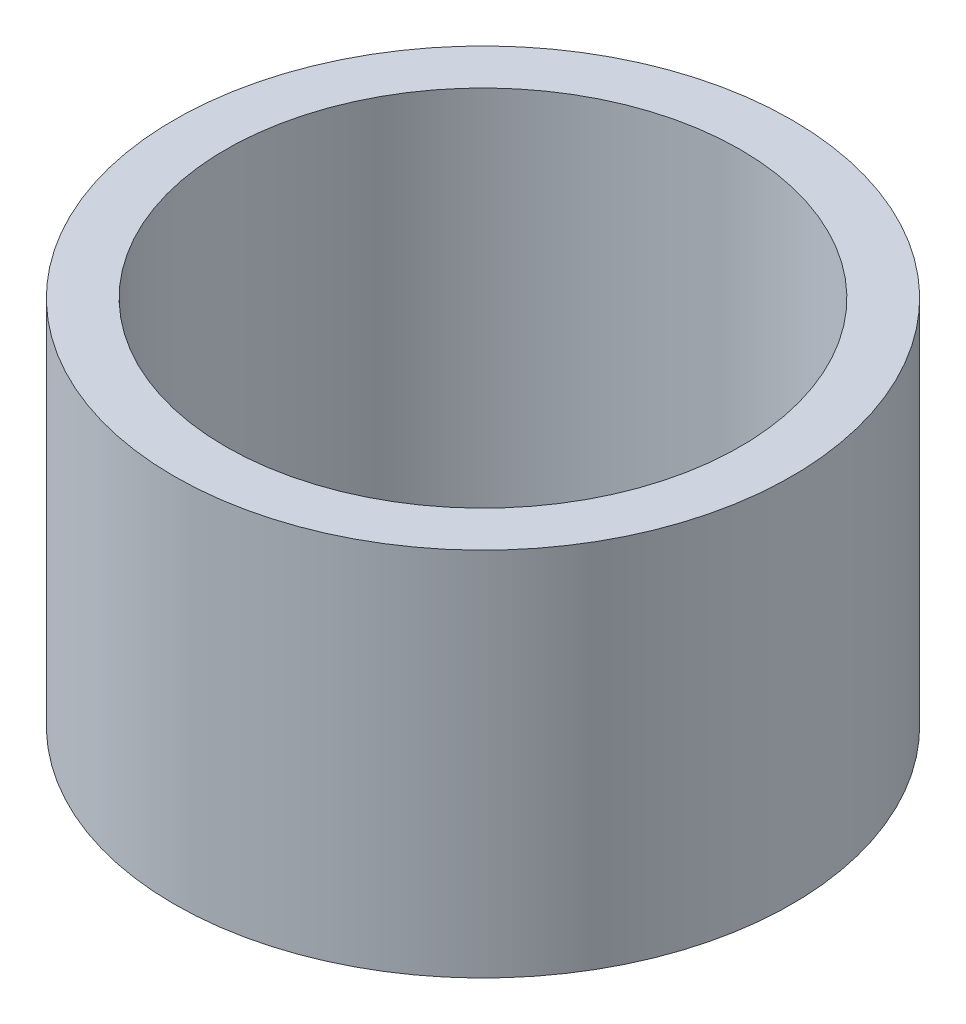
SolidWorks part; units mm, degrees
material "Q235"
ref_plane "Front Plane" through (0, 0, 0) normal (0, 0, 1) x (1, 0, 0)
ref_plane "Top Plane" through (0, 0, 0) normal (0, 1, 0) x (1, 0, 0)
ref_plane "Right Plane" through (0, 0, 0) normal (1, 0, 0) x (0, 0, -1)
sketch "Sketch1" plane through (0, 0, 0) normal (0, 1, 0) x (1, 0, 0)
  circle A1 centre (0, 0) radius 15
  circle A2 centre (0, 0) radius 12.5
  dimension "D1" = 30
  dimension "D2" = 25
extrude "Boss-Extrude1" add sketch "Sketch1" along normal blind 18
